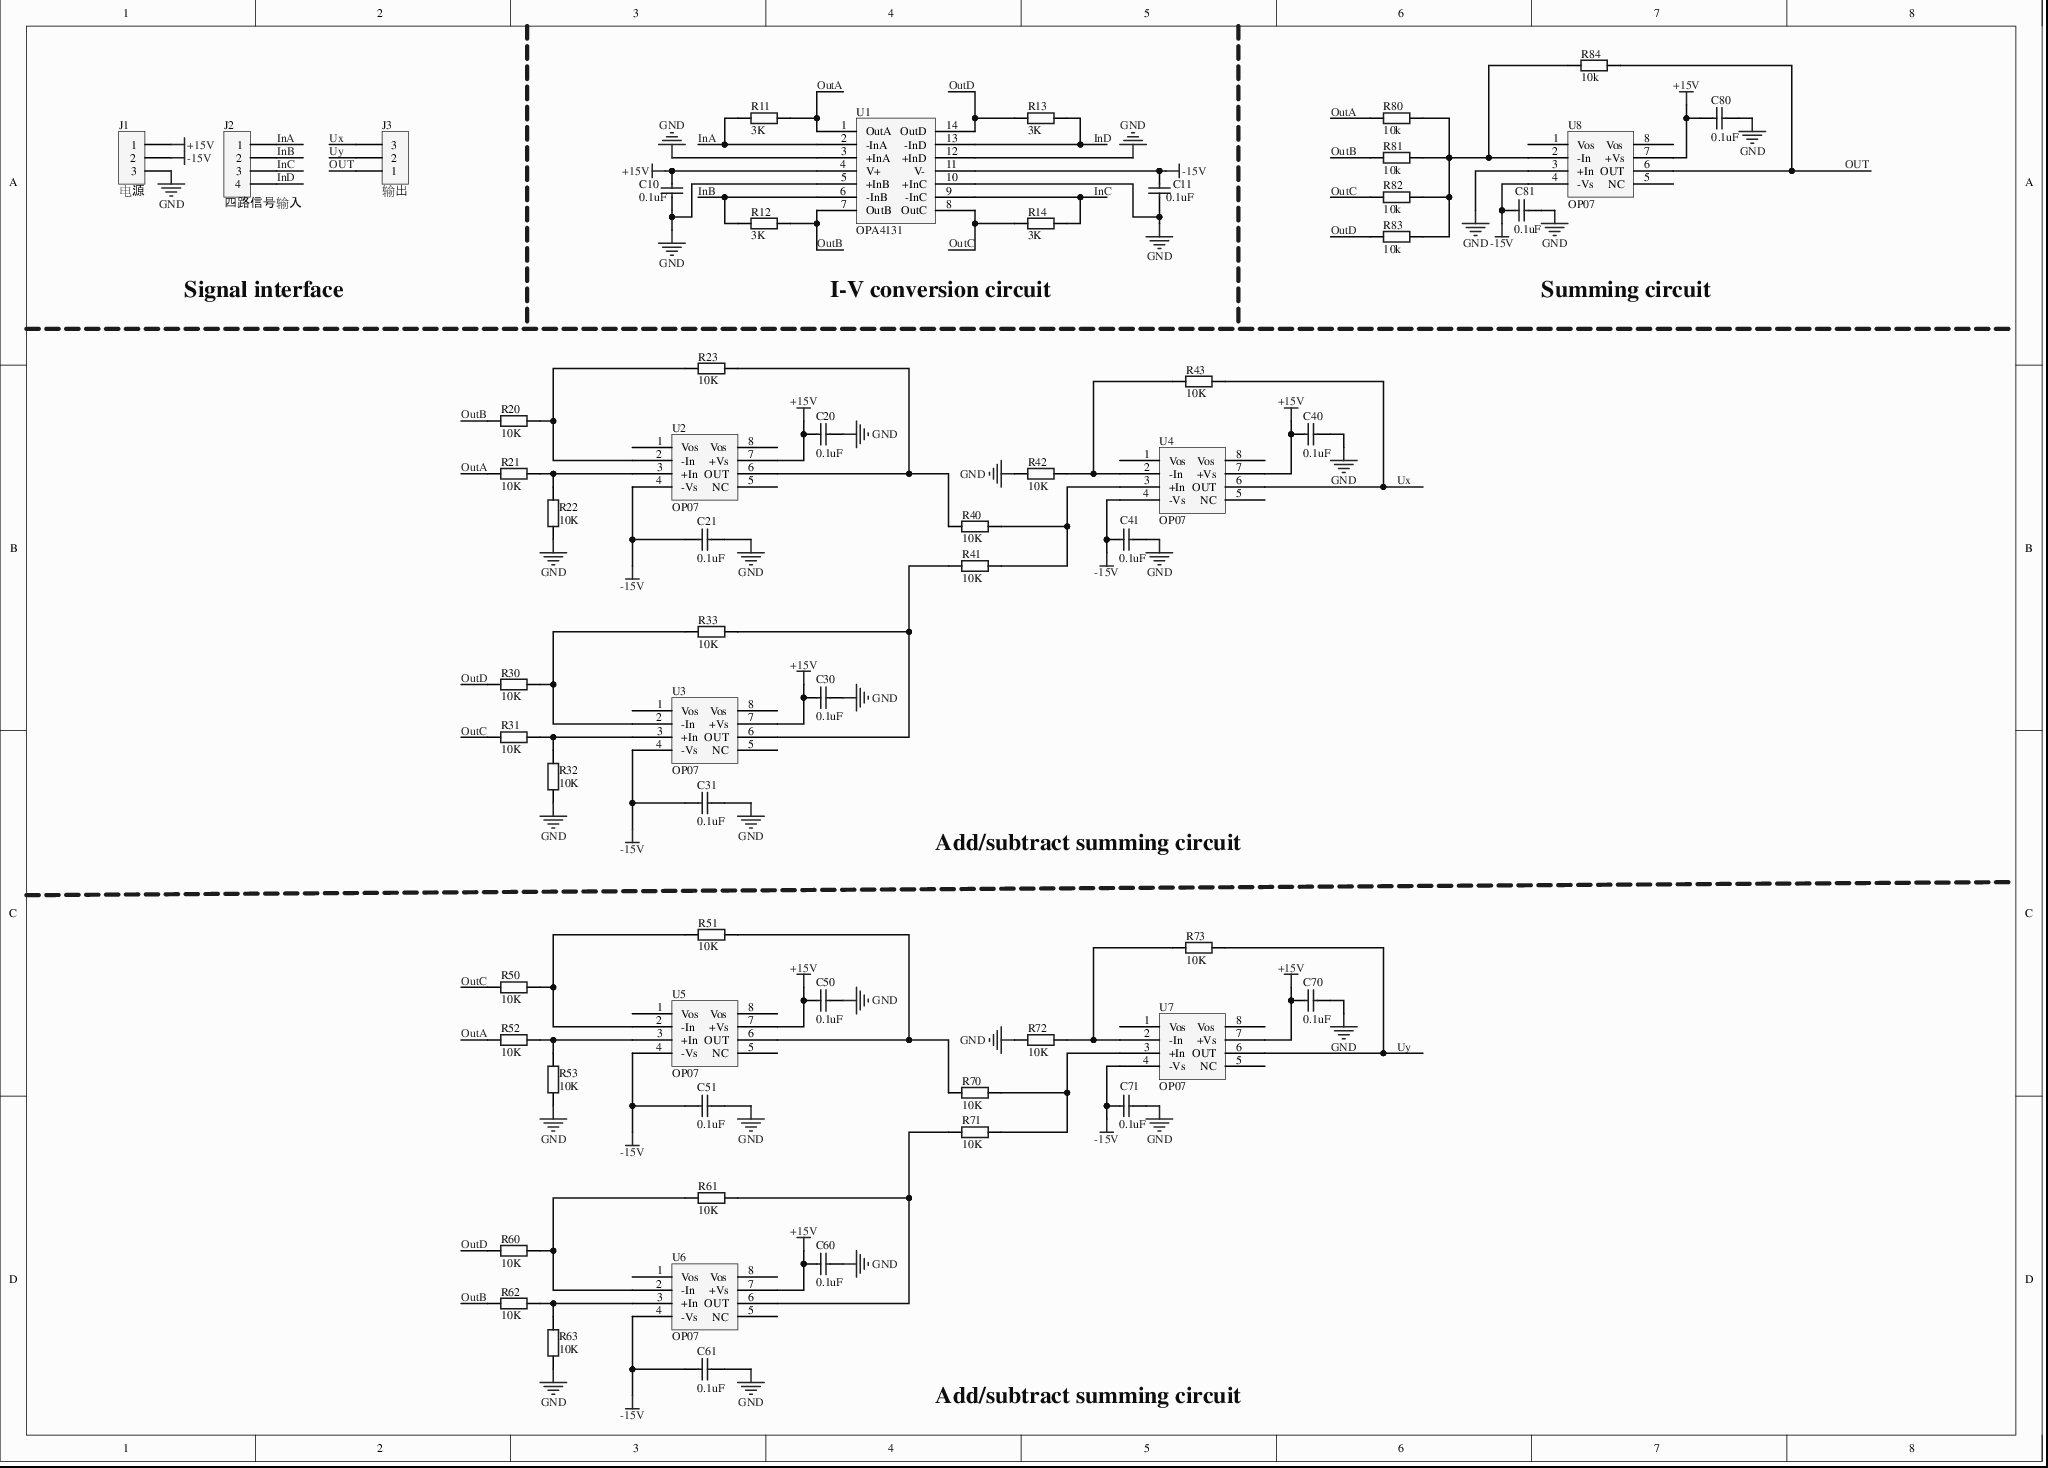
[diagram p0: MISC68795-6.SchDoc]
# Altium project MISC68795-7.PrjPcb
1 sheet, 60 parts. Net scope: global (net labels, ports and power ports of the same name join across sheets).
Board file: MISC68795.PcbDoc

## Sheet MISC68795-6.SchDoc
size A3

### Parts
C10  0.1uF  [C0805]
C11  0.1uF  [C0805]
C20  0.1uF  [C0805]
C21  0.1uF  [C0805]
C30  0.1uF  [C0805]
C31  0.1uF  [C0805]
C40  0.1uF  [C0805]
C41  0.1uF  [C0805]
C50  0.1uF  [C0805]
C51  0.1uF  [C0805]
C60  0.1uF  [C0805]
C61  0.1uF  [C0805]
C70  0.1uF  [C0805]
C71  0.1uF  [C0805]
C80  0.1uF  [C0805]
C81  0.1uF  [C0805]
J1  电源  [HDR1X3]
J2  四路信号输入  [HDR1X4]
J3  输出  [HDR1X3]
R11  3K  [R0805]
R12  3K  [R0805]
R13  3K  [R0805]
R14  3K  [R0805]
R20  10K  [R0805]
R21  10K  [R0805]
R22  10K  [R0805]
R23  10K  [R0805]
R30  10K  [R0805]
R31  10K  [R0805]
R32  10K  [R0805]
R33  10K  [R0805]
R40  10K  [R0805]
R41  10K  [R0805]
R42  10K  [R0805]
R43  10K  [R0805]
R50  10K  [R0805]
R51  10K  [R0805]
R52  10K  [R0805]
R53  10K  [R0805]
R60  10K  [R0805]
R61  10K  [R0805]
R62  10K  [R0805]
R63  10K  [R0805]
R70  10K  [R0805]
R71  10K  [R0805]
R72  10K  [R0805]
R73  10K  [R0805]
R80  10k  [R0805]
R81  10k  [R0805]
R82  10k  [R0805]
R83  10k  [R0805]
R84  10k  [R0805]
U1  OPA4131  [SOIC-14_L8.7-W3.9-P1.27-LS6.0-BL]
U2  OP07  [SOP-8_L4.9-W3.9-P1.27-LS6.0-BL]
U3  OP07  [SOP-8_L4.9-W3.9-P1.27-LS6.0-BL]
U4  OP07  [SOP-8_L4.9-W3.9-P1.27-LS6.0-BL]
U5  OP07  [SOP-8_L4.9-W3.9-P1.27-LS6.0-BL]
U6  OP07  [SOP-8_L4.9-W3.9-P1.27-LS6.0-BL]
U7  OP07  [SOP-8_L4.9-W3.9-P1.27-LS6.0-BL]
U8  OP07  [SOP-8_L4.9-W3.9-P1.27-LS6.0-BL]

### Nets
+15V: C10.2 C20.1 C30.1 C40.1 C50.1 C60.1 C70.1 C80.1 J1.1 U1.4(V+) U2.7(+Vs) U3.7(+Vs) U4.7(+Vs) U5.7(+Vs) U6.7(+Vs) U7.7(+Vs) U8.7(+Vs)
-15V: C11.2 C21.1 C31.1 C41.1 C51.1 C61.1 C71.1 C81.1 J1.2 U1.11(V-) U2.4(-Vs) U3.4(-Vs) U4.4(-Vs) U5.4(-Vs) U6.4(-Vs) U7.4(-Vs) U8.4(-Vs)
GND: C10.1 C11.1 C20.2 C21.2 C30.2 C31.2 C40.2 C41.2 C50.2 C51.2 C60.2 C61.2 C70.2 C71.2 C80.2 C81.2 J1.3 R22.1 R32.1 R42.1 R53.1 R63.1 R72.1 U1.3(+InA) U1.5(+InB) U1.10(+InC) U1.12(+InD) U8.3(+In)
InA: J2.1 R11.1 U1.2(-InA)
InB: J2.2 R12.1 U1.6(-InB)
InC: J2.3 R14.2 U1.9(-InC)
InD: J2.4 R13.2 U1.13(-InD)
OUT: J3.1 R84.2 U8.6(OUT)
OutA: R11.2 R21.1 R52.1 R80.1 U1.1(OutA)
OutB: R12.2 R20.1 R62.1 R81.1 U1.7(OutB)
OutC: R14.1 R31.1 R50.1 R82.1 U1.8(OutC)
OutD: R13.1 R30.1 R60.1 R83.1 U1.14(OutD)
Ux: J3.3 R43.1 U4.6(OUT)
Uy: J3.2 R73.1 U7.6(OUT)
NetR20_2: R20.2 R23.1 U2.2(-In)
NetR21_2: R21.2 R22.2 U2.3(+In)
NetR23_2: R23.2 R40.1 U2.6(OUT)
NetR30_2: R30.2 R33.1 U3.2(-In)
NetR31_2: R31.2 R32.2 U3.3(+In)
NetR33_2: R33.2 R41.1 U3.6(OUT)
NetR40_2: R40.2 R41.2 U4.3(+In)
NetR42_2: R42.2 R43.2 U4.2(-In)
NetR50_2: R50.2 R51.1 U5.2(-In)
NetR51_2: R51.2 R70.1 U5.6(OUT)
NetR52_2: R52.2 R53.2 U5.3(+In)
NetR60_2: R60.2 R61.1 U6.2(-In)
NetR61_2: R61.2 R71.1 U6.6(OUT)
NetR62_2: R62.2 R63.2 U6.3(+In)
NetR70_2: R70.2 R71.2 U7.3(+In)
NetR72_2: R72.2 R73.2 U7.2(-In)
NetR80_2: R80.2 R81.2 R82.2 R83.2 R84.1 U8.2(-In)

Not connected (* = marked no-connect by the designer): U2 1(Vos) 5(NC) 8(Vos); U3 1(Vos) 5(NC) 8(Vos); U4 1(Vos) 5(NC) 8(Vos); U5 1(Vos) 5(NC) 8(Vos); U6 1(Vos) 5(NC) 8(Vos); U7 1(Vos) 5(NC) 8(Vos); U8 1(Vos) 5(NC) 8(Vos)

### Notes on the sheet
- Signal interface
- I-V conversion circuit
- Summing circuit
- Add/subtract summing circuit

### Library data of the parts
C10 C11 C20 C21 C30 C31 C40 C41 C50 C51 C60 C61 C70 C71 C80 C81 = Cap: Capacitor; Value: 100pF; Published: 8-Jun-2000; LatestRevisionDate: 17-Jul-2002; LatestRevisionNote: Re-released for DXP Platform.; PackageReference: RAD-0.3; PackageDescription: Radial Cap, Thru-Hole; 2 Leads; 0.3 in Pin Spacing; Publisher: Altium Limited
J2 = CON4
J3 = 电源
R11-R14 R20-R23 R30-R33 R40-R43 R50-R53 R60-R63 R70-R73 R80-R84 = Res2: Resistor; Value: 1K; Published: 8-Jun-2000; LatestRevisionDate: 17-Jul-2002; LatestRevisionNote: Re-released for DXP Platform.; PackageReference: AXIAL-0.4; PackageDescription: Axial Device, Thru-Hole; 2 Leads; 0.4 in Pin Spacing; Publisher: Altium Limited